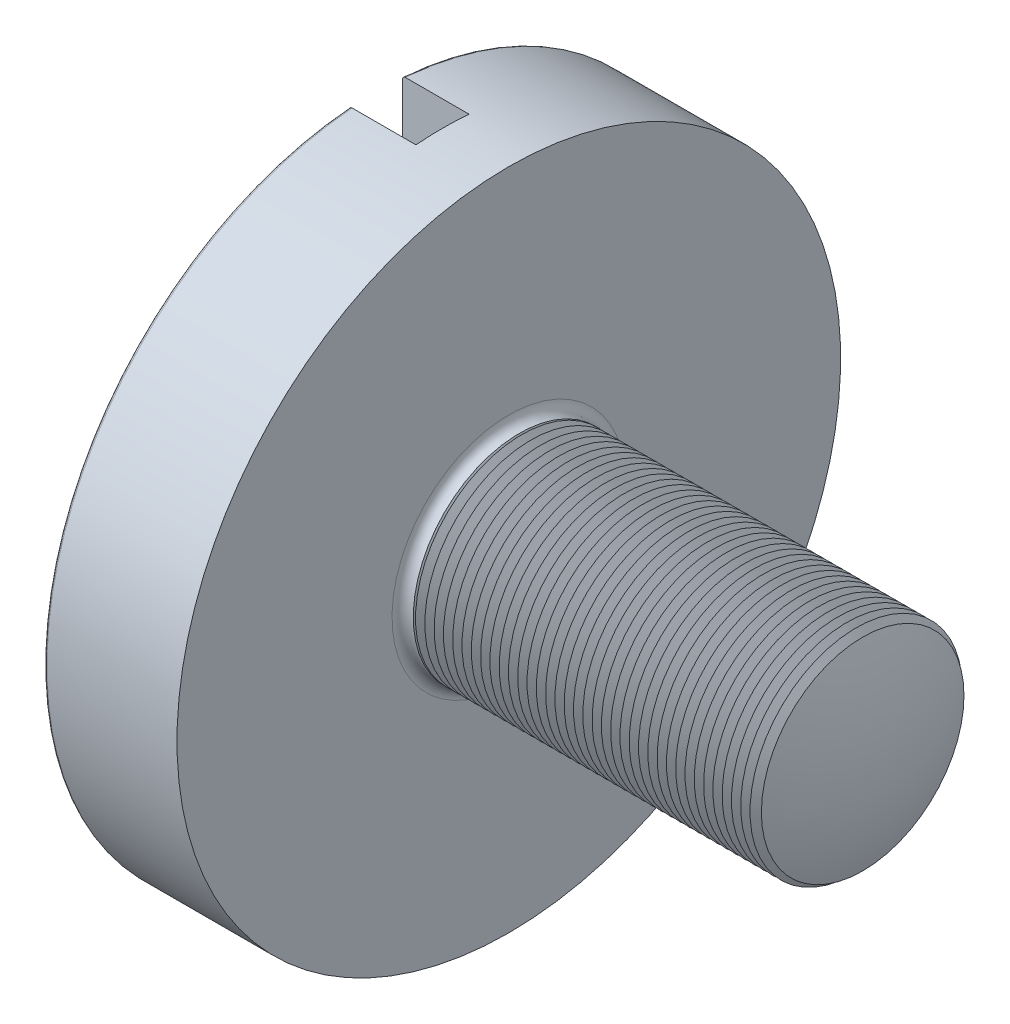
SolidWorks part; units mm, degrees
revolve "基体-旋转" add sketch "草图1" angle 360 about L0
sketch "草图1" plane through (0, 0, 0) normal (0, 0, 1) x (1, 0, 0)
  line L0 (0, 0) -> (4.7398, 0) construction
  line L1 (0, 0) -> (0, 12.5)
  line L2 (0, 12.5) -> (5, 12.5)
  line L3 (5, 12.5) -> (5, 4.4)
  line L4 (5.4, 4) -> (18.2614, 4)
  line L5 (0, 0) -> (19, 0)
  arc A0 (19, 0) -> (18.2614, 4) centre (7.8, 0) ccw
  arc A1 (5.4, 4) -> (5, 4.4) centre (5.4, 4.4) cw
cosmetic thread "装饰螺纹线1" parameters "D1"=13.3, "D2"=7.65
material "33H级"
ref_plane "前视" through (0, 0, 0) normal (0, 0, 1) x (1, 0, 0)
ref_plane "上视" through (0, 0, 0) normal (0, 1, 0) x (1, 0, 0)
ref_plane "右视" through (0, 0, 0) normal (1, 0, 0) x (0, 0, -1)
sketch "尺寸草图" plane through (0, 0, 0) normal (0, 0, 1) x (1, 0, 0)
  line L0 (0, 0) -> (25, 0)
  point P3 (5, 0)
  point P4 (8, 0)
  point P5 (14, 0)
  point P6 (23, 0)
  point P7 (24.6, 0)
  point P8 (22.5, 0)
  point P9 (11.2, 0)
sketch "草图2" plane through (0, 0, 0) normal (-1, 0, 0) x (0, 0, 1)
  line L0 (0, 0) -> (0, -2.5789) construction
  line L3 (1, 12.4599) -> (1, -12.4599)
  line L5 (-1, 12.4599) -> (-1, -12.4599)
  circle A0 centre (0, 0) radius 12.5 construction
  arc A1 (-1, -12.4599) -> (1, -12.4599) centre (0, 0) ccw
  arc A2 (1, 12.4599) -> (-1, 12.4599) centre (0, 0) ccw
extrude "切除-拉伸1" cut sketch "草图2" against normal blind 2.5
fillet "圆角1" radius 0.1 2 edges at (0, 0, -12.5) (0, 0, 12.5)
sketch "草图3" plane through (0, 0, 0) normal (0, 0, 1) x (1, 0, 0)
  line L0 (18.0864, 4) -> (18.4364, 4)
  line L1 (18.4364, 4) -> (18.2614, 3.6969)
  line L2 (18.2614, 3.6969) -> (18.0864, 4)
  line L3 (18.2614, 3.6969) -> (18.2614, 1.9756) construction
  line L5 (18.2614, -4) -> (18.2614, 4) construction
  line L7 (0, 0) -> (-0.7434, 0) construction
revolve "切除-旋转1" cut sketch "草图3" angle 360 about L7
pattern_linear "阵列(线性)1" count 39 spacing 0.35 along (-1, 0, 0) of "切除-旋转1"
equation "\"k@草图1\" = \"k@尺寸草图\""
equation "\"l@草图1\" = \"l@尺寸草图\""
equation "\"r@草图1\" = \"r@尺寸草图\""
equation "\"re@草图1\" = \"re@尺寸草图\""
equation "\"d@草图1\" = \"d@尺寸草图\""
equation "\"dk@草图1\" = \"dk@尺寸草图\""
equation "\"n@草图2\" = \"n@尺寸草图\""
equation "\"t@切除-拉伸1\" = \"t@尺寸草图\""
equation "\"D3@草图3\" = \"d@草图1\" / 2"
equation "\"D1@阵列(线性)1\" =  ( \"l@草图1\" - \"P@阵列(线性)1\" )  / \"P@阵列(线性)1\""
equation "\"D1@装饰螺纹线1\" = \"l@草图1\" - \"P@阵列(线性)1\"*2"
equation "\"D2@装饰螺纹线1\" = \"d@草图1\" - \"P@阵列(线性)1\""
